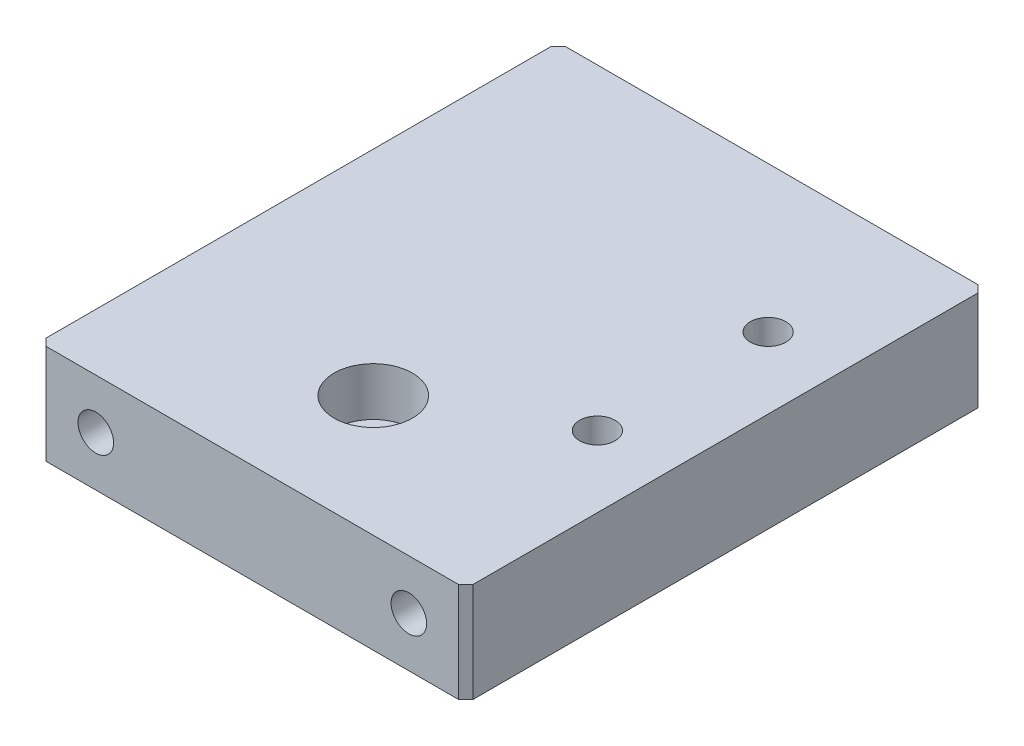
SolidWorks part; units mm, degrees
material "AL6061"
ref_plane "Front Plane" through (0, 0, 0) normal (0, 0, 1) x (1, 0, 0)
ref_plane "Top Plane" through (0, 0, 0) normal (0, 1, 0) x (1, 0, 0)
ref_plane "Right Plane" through (0, 0, 0) normal (1, 0, 0) x (0, 0, -1)
sketch "Sketch1" plane through (0, 0, 0) normal (0, 1, 0) x (1, 0, 0)
  line L1 (-30, -36.5) -> (30, -36.5)
  line L2 (-30, -36.5) -> (-30, 36.5)
  line L3 (-30, 36.5) -> (30, 36.5)
  line L4 (30, -36.5) -> (30, 36.5)
  line L5 (-30, -36.5) -> (30, 36.5) construction
  line L6 (-30, 36.5) -> (30, -36.5) construction
  point P0 (0, 0)
  dimension "D1" = 73
  dimension "D2" = 60
extrude "Boss-Extrude1" add sketch "Sketch1" along normal mid plane 14
hole_wizard "M6 Tapped Hole1" positions "Sketch2" profile "Sketch3" tap size "M6" standard "GB"
sketch "Sketch2" plane through (0, 0, 36.5) normal (0, 0, 1) x (1, 0, 0)
  line L0 (0, 0) -> (0, 11.5764) construction
  line L3 (0, 0) -> (-34.009, 0) construction
  point P13 (-22, 0)
  point P16 (22, 0)
  dimension "D1" = 44
sketch "Sketch3" plane through (22, 0, 36.5) normal (1, 0, 0) x (0, -1, 0)
  line L0 (0, 0) -> (0, 16.5022)
  line L1 (0, 16.5022) -> (2.5, 15)
  line L2 (2.5, 15) -> (2.5, 0)
  line L5 (2.5, 0) -> (0, 0)
  line L10 (0, 16.5022) -> (-2.5, 15) construction
  line L11 (0, -6.35) -> (0, 107.95) construction
  dimension "螺纹孔钻头直径" = 5
  dimension "螺纹孔钻头深度" = 15
  dimension "导头角度" = 118
cosmetic thread "Cosmetic Thread1" parameters "D1"=12, "D2"=6
cosmetic thread "Cosmetic Thread2" parameters "D1"=12, "D2"=6
hole_wizard "M6 Tapped Hole2" positions "Sketch4" profile "Sketch5" tap size "M6" standard "GB" end condition through all
sketch "Sketch4" plane through (0, 7, 0) normal (0, 1, 0) x (1, 0, 0)
  line L0 (20, 31.6624) -> (20, -17.624) construction
  line L1 (-30, -36.5) -> (30, -36.5) construction
  line L2 (30, -36.5) -> (30, 36.5) construction
  point P7 (20, 16)
  point P9 (20, -8)
  dimension "D1" = 24
  dimension "D2" = 28.5
  dimension "D3" = 10
sketch "Sketch5" plane through (20, 7, 8) normal (1, 0, 0) x (0, 0, 1)
  line L0 (0, 0) -> (0, 14)
  line L1 (0, 14) -> (2.5, 14)
  line L2 (2.5, 14) -> (2.5, 0)
  line L5 (2.5, 0) -> (0, 0)
  line L11 (0, -6.35) -> (0, 107.95) construction
  dimension "通孔螺纹孔钻头直径" = 5
  dimension "通孔螺纹孔钻头深度" = 14
cosmetic thread "Cosmetic Thread3" parameters "D2"=6
cosmetic thread "Cosmetic Thread4" parameters "D2"=6
chamfer "Chamfer1" distance 1 angle 45 4 edges at (30, 0, -36.5) (-30, 0, -36.5) (-30, 0, 36.5) (30, 0, 36.5)
hole_wizard "Hole Size per Socket Head Cap Screw Type1" positions "Sketch6" profile "Sketch7" counterbore size "M6" standard "GB" end condition through all
sketch "Sketch6" plane through (0, 7, 0) normal (0, 1, 0) x (1, 0, 0)
  line L0 (0, 0) -> (0, -55.938) construction
  line L1 (-29, -36.5) -> (29, -36.5) construction
  point P7 (0, -19.5)
  dimension "D1" = 17
sketch "Sketch7" plane through (0, 7, 19.5) normal (1, 0, 0) x (0, 0, 1)
  line L0 (0, 0) -> (0, 14)
  line L1 (0, 14) -> (3.3, 14)
  line L3 (3.3, 14) -> (3.3, 6.8)
  line L4 (3.3, 6.8) -> (5.5, 6.8)
  line L5 (5.5, 6.8) -> (5.5, 0)
  line L7 (5.5, 0) -> (0, 0)
  line L11 (0, -6.35) -> (0, 107.95) construction
  dimension "通孔孔直径" = 6.6
  dimension "通孔孔深度" = 14
  dimension "柱形沉头孔直径" = 11
  dimension "柱形沉头孔深度" = 6.8
